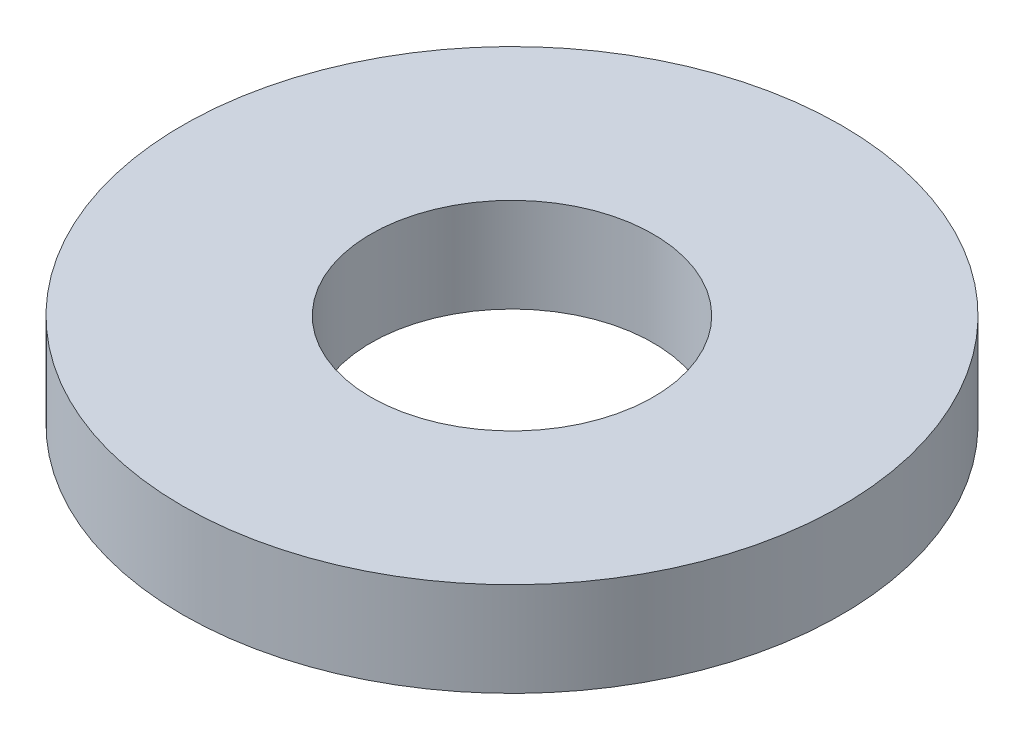
SolidWorks part; units mm, degrees
ref_plane "Front Plane" through (0, 0, 0) normal (0, 0, 1) x (1, 0, 0)
ref_plane "Top Plane" through (0, 0, 0) normal (0, 1, 0) x (1, 0, 0)
ref_plane "Right Plane" through (0, 0, 0) normal (1, 0, 0) x (0, 0, -1)
sketch "Sketch1" plane through (0, 0, 0) normal (0, 1, 0) x (1, 0, 0)
  circle A0 centre (0, 0) radius 5.25
  circle A1 centre (0, 0) radius 2.25
  point P0 (0, 0)
  dimension "D3" = 4.5
  dimension "D4" = 10.5
extrude "Boss-Extrude1" add sketch "Sketch1" along normal blind 1.5
